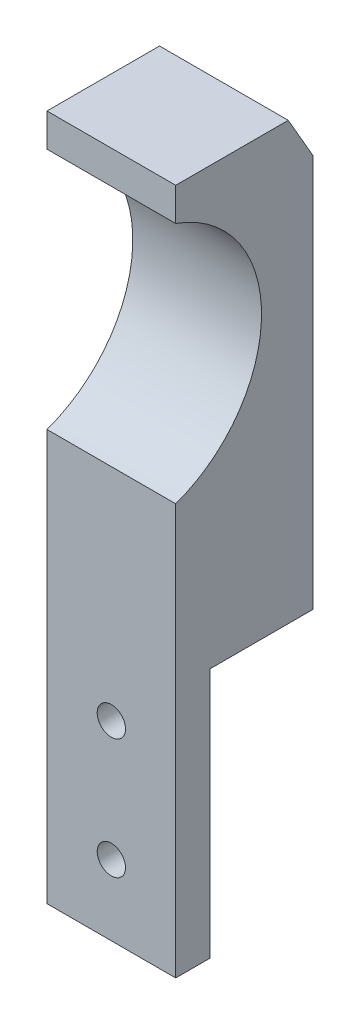
SolidWorks part; units mm, degrees
material "1060 合金"
ref_plane "Front Plane" through (0, 0, 0) normal (0, 0, 1) x (1, 0, 0)
ref_plane "Top Plane" through (0, 0, 0) normal (0, 1, 0) x (1, 0, 0)
ref_plane "Right Plane" through (0, 0, 0) normal (1, 0, 0) x (0, 0, -1)
sketch "Sketch1" plane through (0, 0, 0) normal (0, 0, 1) x (1, 0, 0)
  line L1 (-7.5, -40) -> (7.5, -40)
  line L2 (-7.5, -40) -> (-7.5, 40)
  line L3 (-7.5, 40) -> (7.5, 40)
  line L4 (7.5, -40) -> (7.5, 40)
  line L5 (-7.5, -40) -> (7.5, 40) construction
  line L6 (-7.5, 40) -> (7.5, -40) construction
  point P0 (0, 0)
  dimension "D1" = 15
  dimension "D2" = 80
extrude "Boss-Extrude1" add sketch "Sketch1" along normal blind 16
sketch "Sketch2" plane through (7.5, 0, 0) normal (1, 0, 0) x (0, 0, -1)
  line L0 (-16, -40) -> (0, -40) construction
  line L1 (-12, -40) -> (0, -40)
  line L2 (-12, -40) -> (-12, -10.8)
  line L3 (-12, -10.8) -> (0, -10.8)
  line L4 (0, -40) -> (0, -10.8)
  line L5 (0, -40) -> (0, 40) construction
  dimension "D1" = 12
  dimension "D2" = 29.2
extrude "Cut-Extrude1" cut sketch "Sketch2" against normal through all
hole_wizard "M4 Tapped Hole1" positions "Sketch3" profile "Sketch4" tap size "M4" standard "ISO"
sketch "Sketch3" plane through (0, 0, 12) normal (0, 0, -1) x (-1, 0, 0)
  line L0 (7.5, -40) -> (-7.5, -40) construction
  point P0 (0, -17.8)
  point P2 (0, -31.8)
  dimension "D1" = 14
  dimension "D2" = 8.2
sketch "Sketch4" plane through (0, -17.8, 12) normal (1, 0, 0) x (0, 1, 0)
  line L0 (0, 0) -> (0, 23.2414)
  line L1 (0, 23.2414) -> (1.65, 22.25)
  line L2 (1.65, 22.25) -> (1.65, 0)
  line L5 (1.65, 0) -> (0, 0)
  line L10 (0, 23.2414) -> (-1.65, 22.25) construction
  line L11 (0, -6.35) -> (0, 107.95) construction
  dimension "螺纹孔钻头直径" = 3.3
  dimension "螺纹孔钻头深度" = 22.25
  dimension "导头角度" = 118
cosmetic thread "Cosmetic thread1" parameters "D1"=8, "D2"=4
cosmetic thread "Cosmetic thread2" parameters "D1"=8, "D2"=4
chamfer "Chamfer1" distance 5 angle 30 1 edges at (0, 40, 0)
sketch "Sketch6" plane through (7.5, 0, 0) normal (1, 0, 0) x (0, 0, -1)
  line L0 (-16, -40) -> (-16, 40) construction
  line L1 (-16, 40) -> (-2.8868, 40) construction
  circle A0 centre (-21, 22) radius 15
  dimension "D2" = 30
  dimension "D1" = 5
  dimension "D3" = 18
extrude "Cut-Extrude2" cut sketch "Sketch6" against normal through all
